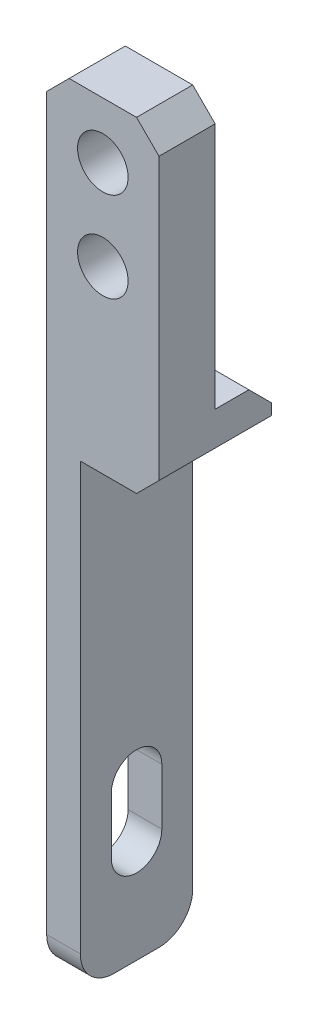
SolidWorks part; units mm, degrees
material "S45C"
ref_plane "Front Plane" through (0, 0, 0) normal (0, 0, 1) x (1, 0, 0)
ref_plane "Top Plane" through (0, 0, 0) normal (0, 1, 0) x (1, 0, 0)
ref_plane "Right Plane" through (0, 0, 0) normal (1, 0, 0) x (0, 0, -1)
sketch "Sketch1" plane through (0, 0, 0) normal (0, 0, 1) x (1, 0, 0)
  line L1 (-5, -35) -> (5, -35)
  line L2 (-5, -35) -> (-5, 35)
  line L3 (-5, 35) -> (5, 35)
  line L4 (5, -35) -> (5, 35)
  line L5 (-5, -35) -> (5, 35) construction
  line L6 (-5, 35) -> (5, -35) construction
  point P0 (0, 0)
  dimension "D1" = 10
  dimension "D2" = 70
extrude "Boss-Extrude1" add sketch "Sketch1" along normal mid plane 10
sketch "Sketch2" plane through (0, 0, 5) normal (0, 0, 1) x (1, 0, 0)
  line L0 (-5, 35) -> (-5, -35) construction
  line L1 (5, -35) -> (-2, -35)
  line L2 (5, -35) -> (5, 6)
  line L3 (5, 6) -> (-2, 6)
  line L4 (-2, -35) -> (-2, 6)
  dimension "D1" = 41
  dimension "D2" = 3
extrude "Cut-Extrude1" cut sketch "Sketch2" against normal through all
sketch "Sketch3" plane through (5, 0, 0) normal (1, 0, 0) x (0, 0, -1)
  line L0 (-5, 6) -> (-5, 35) construction
  line L1 (5, 35) -> (0, 35)
  line L2 (5, 35) -> (5, 11)
  line L3 (5, 11) -> (0, 11)
  line L4 (0, 35) -> (0, 11)
  dimension "D1" = 5
  dimension "D2" = 24
extrude "Cut-Extrude2" cut sketch "Sketch3" against normal through all
sketch "Sketch4" plane through (-5, 0, 0) normal (-1, 0, 0) x (0, 0, 1)
  line L0 (0, -21) -> (0, -26) construction
  line L1 (2.25, -21) -> (2.25, -26)
  line L2 (-2.25, -21) -> (-2.25, -26)
  line L3 (5, -35) -> (-5, -35) construction
  arc A0 (2.25, -21) -> (-2.25, -21) centre (0, -21) ccw
  arc A1 (-2.25, -26) -> (2.25, -26) centre (0, -26) ccw
  point P3 (0, -23.5)
  dimension "D3" = 2.25
  dimension "D1" = 5
  dimension "D2" = 11.5
extrude "Cut-Extrude3" cut sketch "Sketch4" against normal through all
fillet "Fillet1" radius 3 2 edges at (-3.5, -35, -5) (-3.5, -35, 5)
hole_wizard "M4 Clearance Hole1" positions "Sketch6" profile "Sketch5" hole size "M4" standard "GB" end condition through all
sketch "Sketch6" plane through (0, 0, 5) normal (0, 0, 1) x (1, 0, 0)
  line L0 (5, 35) -> (-5, 35) construction
  point P0 (0, 30)
  point P2 (0, 22)
  dimension "D1" = 5
  dimension "D2" = 8
sketch "Sketch5" plane through (0, 30, 5) normal (1, 0, 0) x (0, -1, 0)
  line L0 (0, 0) -> (0, 10)
  line L1 (0, 10) -> (2.25, 10)
  line L2 (2.25, 10) -> (2.25, 0)
  line L5 (2.25, 0) -> (0, 0)
  line L11 (0, -6.35) -> (0, 107.95) construction
  dimension "通孔孔直径" = 4.5
  dimension "通孔孔深度" = 10
chamfer "Chamfer1" distance 2 angle 45 4 edges at (5, 6, 0) (0, 11, -5) (-5, 35, 2.5) (5, 35, 2.5)
